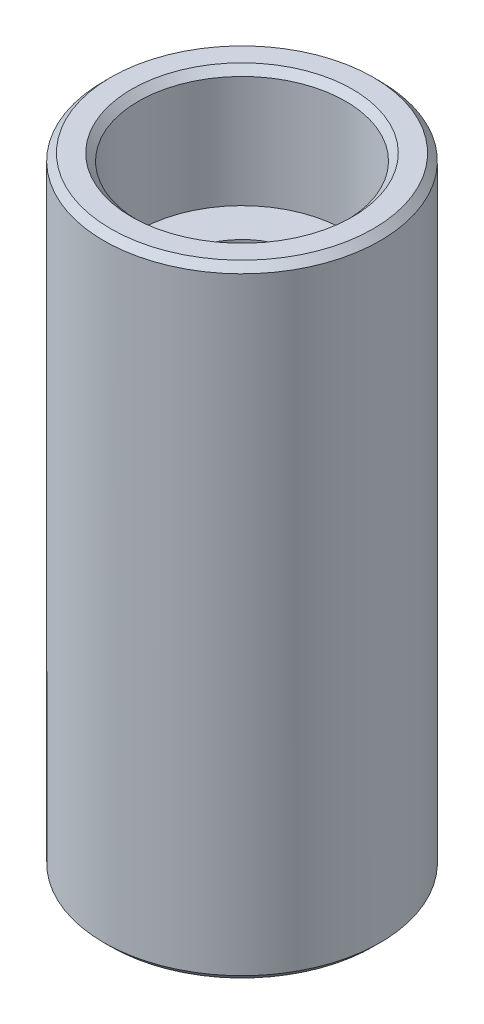
from build123d import *

# Parameters (mm, degrees)
SKETCH1_R                                           = 10
BOSS_EXTRUDE1_DEPTH                                 = 45
CBORE_FOR_M8_HEX_SOCKET_HEAD_CAP_SCREW1_D           = 9
CBORE_FOR_M8_HEX_SOCKET_HEAD_CAP_SCREW1_CBORE_D     = 15
CBORE_FOR_M8_HEX_SOCKET_HEAD_CAP_SCREW1_CBORE_DEPTH = 8.6
CHAMFER1_SIZE                                       = 0.5


with BuildPart() as part:
    # Sketch1 → Boss-Extrude1 (new body)
    with BuildSketch(Plane(origin=(0, 0, 0), x_dir=(1, 0, 0), z_dir=(0, 1, 0))):
        with Locations(Location((0, 0, 0), (0, 0, 90))):
            Circle(SKETCH1_R)
    extrude(amount=BOSS_EXTRUDE1_DEPTH)

    # CBORE for M8 Hex Socket Head Cap Screw1 (through all)
    with Locations(Plane(origin=(0, 45, 0), x_dir=(1, 0, 0), z_dir=(0, 1, 0))):
        with Locations((0, 0)):
            CounterBoreHole(CBORE_FOR_M8_HEX_SOCKET_HEAD_CAP_SCREW1_D / 2, CBORE_FOR_M8_HEX_SOCKET_HEAD_CAP_SCREW1_CBORE_D / 2, CBORE_FOR_M8_HEX_SOCKET_HEAD_CAP_SCREW1_CBORE_DEPTH)

    # Chamfer1
    chamfer1_edges = [part.edges().sort_by_distance(p)[0] for p in [
        (0, 0, 10),
        (0, 45, 10),
        (-7.5, 45, 0),
        (4.5, 0, 0),
    ]]
    chamfer(chamfer1_edges, length=CHAMFER1_SIZE)


solid = part.part
